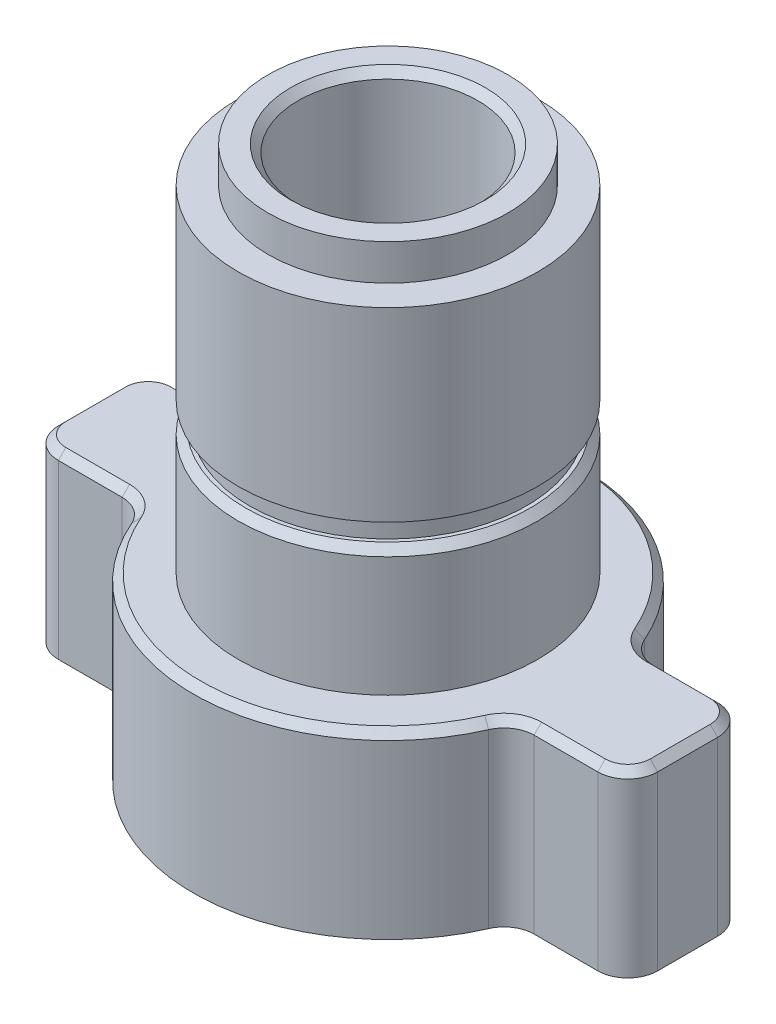
SolidWorks part; units mm, degrees
other "标注1"
sketch "草图10" plane through (-10, 18.4, 6.5) normal (-0.568, 0.1721, 0.8049) x (0.1294, 0.9844, -0.1192)
material "AISI 304"
ref_plane "前视基准面" through (0, 0, 0) normal (0, 0, 1) x (1, 0, 0)
ref_plane "上视基准面" through (0, 0, 0) normal (0, 1, 0) x (1, 0, 0)
ref_plane "右视基准面" through (0, 0, 0) normal (1, 0, 0) x (0, 0, -1)
sketch "草图1" plane through (0, 0, 0) normal (0, 1, 0) x (1, 0, 0)
  line L0 (6.8739, 2) -> (9, 2)
  line L1 (10, 1) -> (10, -1)
  line L2 (9, -2) -> (6.8739, -2)
  line L3 (2.5287, 0) -> (50002.5287, 0) construction
  line L4 (0, 6.5) -> (0, -6.5) construction
  line L5 (-10, 1) -> (-10, -1)
  line L6 (-9, -2) -> (-6.8739, -2)
  line L7 (-6.8739, 2) -> (-9, 2)
  arc A0 (-5.9573, -2.6) -> (5.9573, -2.6) centre (0, 0) ccw
  arc A2 (10, -1) -> (9, -2) centre (9, -1) cw
  arc A3 (9, 2) -> (10, 1) centre (9, 1) cw
  arc A4 (-9, 2) -> (-10, 1) centre (-9, 1) ccw
  arc A5 (-10, -1) -> (-9, -2) centre (-9, -1) ccw
  arc A6 (5.9573, 2.6) -> (-5.9573, 2.6) centre (0, 0) ccw
  arc A7 (6.8739, 2) -> (5.9573, 2.6) centre (6.8739, 3) cw
  arc A8 (6.8739, -2) -> (5.9573, -2.6) centre (6.8739, -3) ccw
  arc A9 (-6.8739, -2) -> (-5.9573, -2.6) centre (-6.8739, -3) cw
  arc A10 (-6.8739, 2) -> (-5.9573, 2.6) centre (-6.8739, 3) ccw
  point P25 (6.1847, 2)
  point P28 (6.1847, -2)
  point P31 (-6.1847, -2)
  point P34 (-6.1847, 2)
  dimension "D2" = 13
  dimension "D4" = 1
  dimension "D6" = 1
  dimension "D3" = 4
  dimension "D5" = 20
extrude "凸台-拉伸1" add sketch "草图1" along normal blind 6
sketch "草图2" plane through (0, 6, 0) normal (0, 1, 0) x (1, 0, 0)
  circle A0 centre (0, 0) radius 5
  dimension "D1" = 10
extrude "凸台-拉伸2" add sketch "草图2" along normal blind 4.25
sketch "草图3" plane through (0, 10.25, 0) normal (0, 1, 0) x (1, 0, 0)
  circle A0 centre (0, 0) radius 4.625
  dimension "D1" = 9.25
extrude "凸台-拉伸3" add sketch "草图3" along normal blind 0.75
sketch "草图4" plane through (0, 11, 0) normal (0, 1, 0) x (1, 0, 0)
  circle A1 centre (0, 0) radius 5 construction
  circle A3 centre (0, 0) radius 5
extrude "M10×1 细牙螺柱" add sketch "草图4" along normal blind 6.2
sketch "草图5" plane through (0, 17.2, 0) normal (0, 1, 0) x (1, 0, 0)
  circle A0 centre (0, 0) radius 4
  dimension "D1" = 8
extrude "凸台-拉伸5" add sketch "草图5" along normal blind 1.2
sketch "草图6" plane through (0, 18.4, 0) normal (0, 1, 0) x (1, 0, 0)
  circle A0 centre (0, 0) radius 3
  dimension "D1" = 6
extrude "切除-拉伸1" cut sketch "草图6" against normal blind 5
hole_wizard "M5 螺纹孔1" positions "草图9" profile "草图8" tap size "M5" standard "GB" end condition through all
sketch "草图9" plane through (0, 0, 0) normal (0, -1, 0) x (-1, 0, 0)
  point P0 (0, 0)
sketch "草图8" plane through (0, 0, 0) normal (1, 0, 0) x (0, 0, -1)
  line L0 (0, 0) -> (0, 18.4)
  line L1 (0, 18.4) -> (2.1, 18.4)
  line L2 (2.1, 18.4) -> (2.1, 0)
  line L5 (2.1, 0) -> (0, 0)
  line L11 (0, -6.35) -> (0, 107.95) construction
  dimension "通孔螺纹孔钻头直径" = 4.2
  dimension "通孔螺纹孔钻头深度" = 18.4
cosmetic thread "孔螺纹线1" parameters "D2"=5
chamfer "C0.25 倒角1" distance 0.25 angle 45 18 edges at (0, 18.4, 3) (0, 10.25, 5) (0, 6, 6.5) (6.3261, 6, 2.1633) (-6.3261, 6, 2.1633) (7.9369, 6, 2) (-7.9369, 6, 2) (9.7071, 6, 1.7071) (-9.7071, 6, 1.7071) (10, 6, 0) (-10, 6, 0) (9.7071, 6, -1.7071) (-9.7071, 6, -1.7071) (7.9369, 6, -2) (-7.9369, 6, -2) (6.3261, 6, -2.1633) (-6.3261, 6, -2.1633) (0, 6, -6.5)
